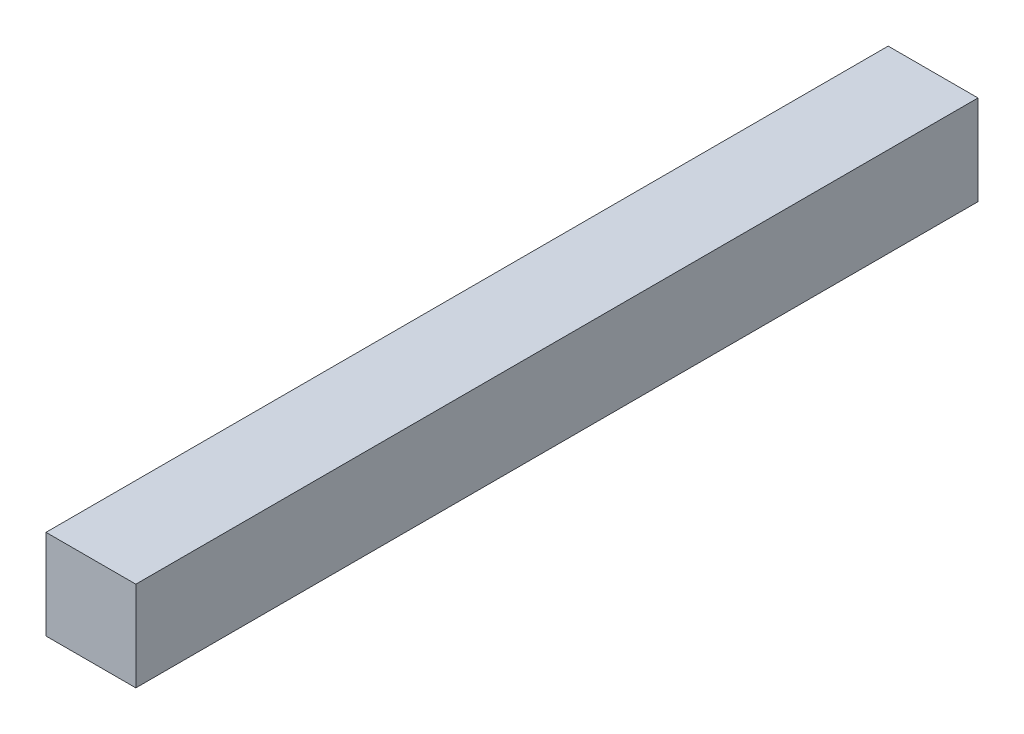
from build123d import *

# Parameters (mm, degrees)
SKETCH_1_W      = 16
SKETCH_1_H      = 16
EXTRUDE_1_DEPTH = 150


with BuildPart() as part:
    # 草图1 → 凸台-拉伸1 (new body)
    with BuildSketch(Plane.XY):
        Rectangle(SKETCH_1_W, SKETCH_1_H)
    extrude(amount=EXTRUDE_1_DEPTH)


solid = part.part
